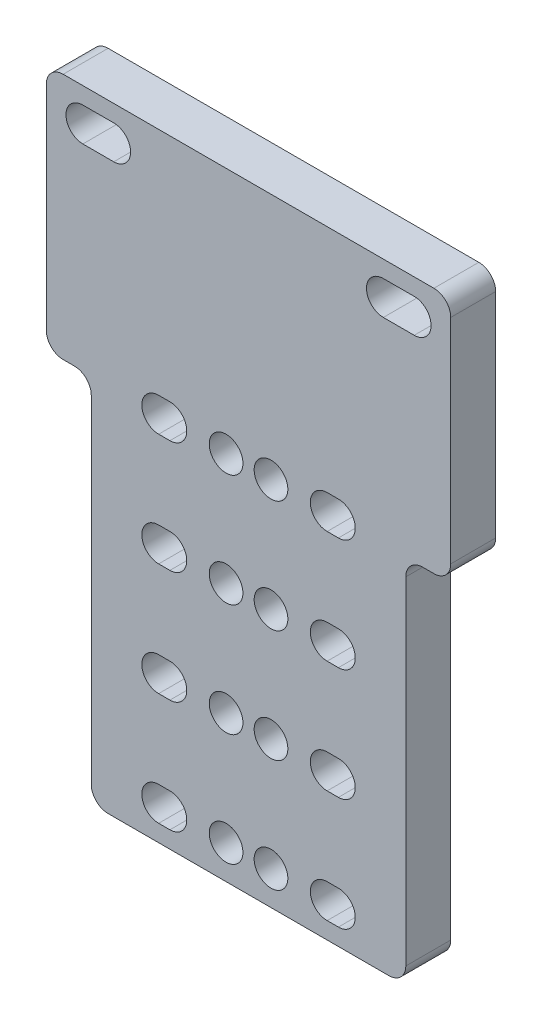
from build123d import *

# Parameters (mm, degrees)
SKETCH1_W           = 36
SKETCH1_H           = 55
BOSS_EXTRUDE1_DEPTH = 4
SKETCH2_R           = 1.5
CUT_EXTRUDE1_DEPTH  = 4
FILLET1_R           = 1.5
BOSS_EXTRUDE2_DEPTH = 4


with BuildPart() as part:
    # Sketch1 → Boss-Extrude1 (new body)
    with BuildSketch(Plane.XY):
        Rectangle(SKETCH1_W, SKETCH1_H)
    extrude(amount=BOSS_EXTRUDE1_DEPTH)

    # Sketch2 → Cut-Extrude1 (cut)
    with BuildSketch(Plane.XY.offset(4)):
        with BuildLine():
            Line((-14.75, 23), (-12, 23))
            ThreePointArc((-12, 23), (-10.5, 24.5), (-12, 26))
            Line((-12, 26), (-14.75, 26))
            ThreePointArc((-14.75, 26), (-16.25, 24.5), (-14.75, 23))
        make_face()
        with BuildLine():
            Line((12, 23), (14.75, 23))
            ThreePointArc((14.75, 23), (16.25, 24.5), (14.75, 26))
            Line((14.75, 26), (12, 26))
            ThreePointArc((12, 26), (10.5, 24.5), (12, 23))
        make_face()
        with BuildLine():
            Line((-8, 4), (-7, 4))
            ThreePointArc((-7, 4), (-5.5, 5.5), (-7, 7))
            Line((-7, 7), (-8, 7))
            ThreePointArc((-8, 7), (-9.5, 5.5), (-8, 4))
        make_face()
        with Locations((-2, 5.5)):
            Circle(SKETCH2_R)
        with Locations((2, 5.5)):
            Circle(SKETCH2_R)
        with BuildLine():
            Line((7, 4), (8, 4))
            ThreePointArc((8, 4), (9.5, 5.5), (8, 7))
            Line((8, 7), (7, 7))
            ThreePointArc((7, 7), (5.5, 5.5), (7, 4))
        make_face()
        with BuildLine():
            Line((7, -6), (8, -6))
            ThreePointArc((8, -6), (9.5, -4.5), (8, -3))
            Line((8, -3), (7, -3))
            ThreePointArc((7, -3), (5.5, -4.5), (7, -6))
        make_face()
        with Locations((2, -4.5)):
            Circle(SKETCH2_R)
        with Locations((-2, -4.5)):
            Circle(SKETCH2_R)
        with BuildLine():
            Line((-8, -6), (-7, -6))
            ThreePointArc((-7, -6), (-5.5, -4.5), (-7, -3))
            Line((-7, -3), (-8, -3))
            ThreePointArc((-8, -3), (-9.5, -4.5), (-8, -6))
        make_face()
        with BuildLine():
            Line((-8, -16), (-7, -16))
            ThreePointArc((-7, -16), (-5.5, -14.5), (-7, -13))
            Line((-7, -13), (-8, -13))
            ThreePointArc((-8, -13), (-9.5, -14.5), (-8, -16))
        make_face()
        with BuildLine():
            Line((-8, -26), (-7, -26))
            ThreePointArc((-7, -26), (-5.5, -24.5), (-7, -23))
            Line((-7, -23), (-8, -23))
            ThreePointArc((-8, -23), (-9.5, -24.5), (-8, -26))
        make_face()
        with Locations((-2, -14.5)):
            Circle(SKETCH2_R)
        with Locations((-2, -24.5)):
            Circle(SKETCH2_R)
        with Locations((2, -14.5)):
            Circle(SKETCH2_R)
        with Locations((2, -24.5)):
            Circle(SKETCH2_R)
        with BuildLine():
            Line((7, -26), (8, -26))
            ThreePointArc((8, -26), (9.5, -24.5), (8, -23))
            Line((8, -23), (7, -23))
            ThreePointArc((7, -23), (5.5, -24.5), (7, -26))
        make_face()
        Polygon((-14, 5.5), (-18, 5.5), (-18, -26), (-18, -27.5), (-16.5, -27.5), (-14, -27.5), align=None)
        Polygon((14, 5.5), (14, -27.5), (16.5, -27.5), (18, -27.5), (18, -26), (18, 5.5), align=None)
        with BuildLine():
            ThreePointArc((7, -13), (5.5, -14.5), (7, -16))
            Line((7, -16), (8, -16))
            ThreePointArc((8, -16), (9.5, -14.5), (8, -13))
            Line((8, -13), (7, -13))
        make_face()
    extrude(amount=-CUT_EXTRUDE1_DEPTH, mode=Mode.SUBTRACT)

    # Fillet1
    fillet1_edges = [part.edges().sort_by_distance(p)[0] for p in [
        (18, 5.5, 2),
        (14, -27.5, 2),
        (-14, -27.5, 2),
        (-18, 5.5, 2),
        (-18, 27.5, 2),
        (18, 27.5, 2),
    ]]
    fillet(fillet1_edges, radius=FILLET1_R)

    # Sketch3 → Boss-Extrude2 (add)
    with BuildSketch(Plane.XY.offset(4)):
        with BuildLine():
            Line((-14, 5.5), (-14, 4))
            ThreePointArc((-14, 4), (-14.439339828, 5.060660172), (-15.5, 5.5))
            Line((-15.5, 5.5), (-14, 5.5))
        make_face()
        with BuildLine():
            ThreePointArc((15.5, 5.5), (14.439339828, 5.060660172), (14, 4))
            Line((14, 4), (14, 5.5))
            Line((14, 5.5), (15.5, 5.5))
        make_face()
    extrude(amount=-BOSS_EXTRUDE2_DEPTH)


solid = part.part
